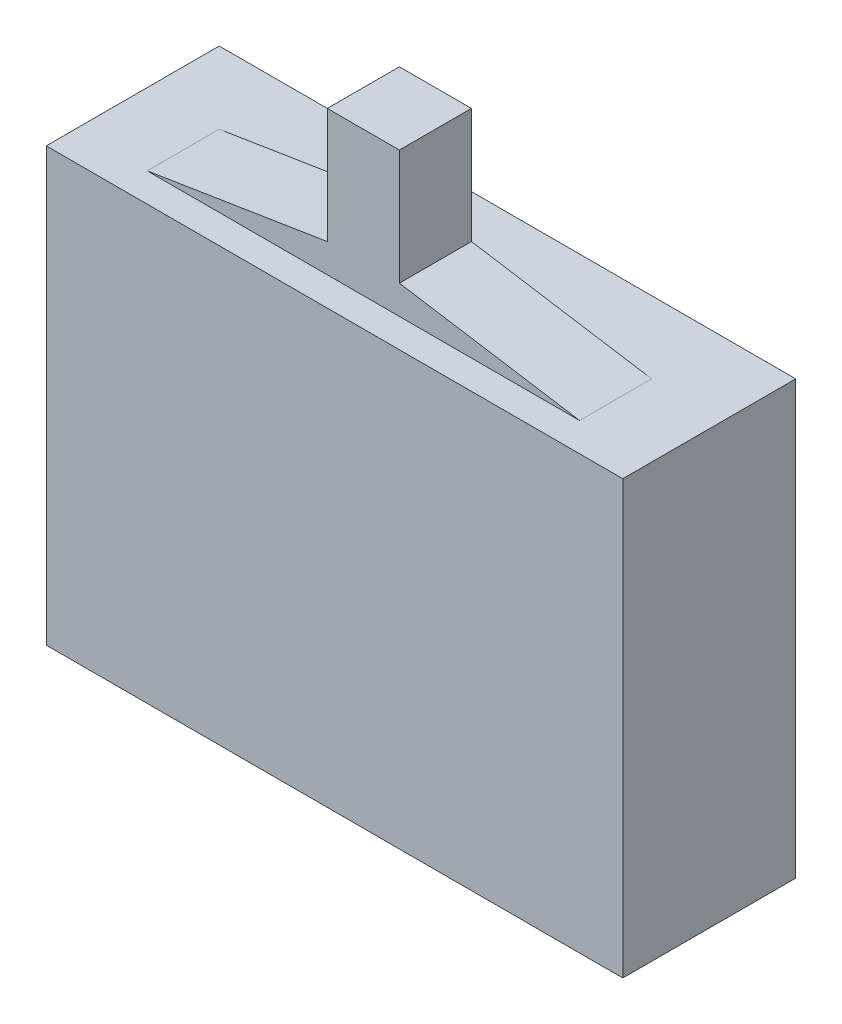
from build123d import *

# Parameters (mm, degrees)
SKETCH1_W           = 40
SKETCH1_H           = 30
BOSS_EXTRUDE1_DEPTH = 12
BOSS_EXTRUDE3_START = 5
BOSS_EXTRUDE3_DEPTH = 5


with BuildPart() as part:
    # Sketch1 → Boss-Extrude1 (new body)
    with BuildSketch(Plane.XY):
        with Locations((20, -15)):
            Rectangle(SKETCH1_W, SKETCH1_H)
    extrude(amount=BOSS_EXTRUDE1_DEPTH)

    # Sketch2 → Boss-Extrude3 (add)
    with BuildSketch(Plane.XY.offset(BOSS_EXTRUDE3_START)):
        Polygon((17.5, 10), (17.5, 2), (5, 0), (35, 0), (22.5, 2), (22.5, 10), align=None)
    extrude(amount=BOSS_EXTRUDE3_DEPTH)


solid = part.part
